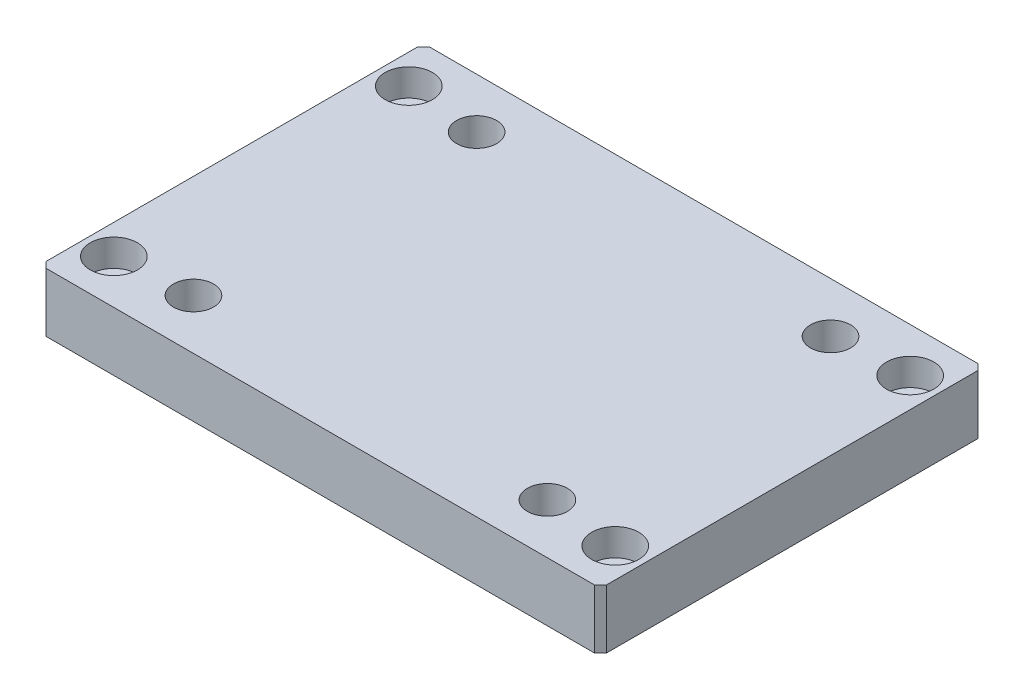
SolidWorks part; units mm, degrees
material "A6061"
ref_plane "前基準面" through (0, 0, 0) normal (0, 0, 1) x (1, 0, 0)
ref_plane "上基準面" through (0, 0, 0) normal (0, 1, 0) x (1, 0, 0)
ref_plane "右基準面" through (0, 0, 0) normal (1, 0, 0) x (0, 0, -1)
sketch "草图1" plane through (0, 0, 0) normal (0, 1, 0) x (1, 0, 0)
  line L1 (-47.5, -32.5) -> (47.5, -32.5)
  line L2 (-47.5, -32.5) -> (-47.5, 32.5)
  line L3 (-47.5, 32.5) -> (47.5, 32.5)
  line L4 (47.5, -32.5) -> (47.5, 32.5)
  line L5 (-47.5, -32.5) -> (47.5, 32.5) construction
  line L6 (-47.5, 32.5) -> (47.5, -32.5) construction
  point P0 (0, 0)
  dimension "D1" = 95
  dimension "D2" = 65
extrude "凸台-拉伸1" add sketch "草图1" along normal mid plane 10
chamfer "倒角1" distance 1 angle 45 4 edges at (47.5, 0, -32.5) (47.5, 0, 32.5) (-47.5, 0, 32.5) (-47.5, 0, -32.5)
sketch "草图2" plane through (0, 5, 0) normal (0, 1, 0) x (1, 0, 0)
  line L0 (0, 50.3233) -> (0, 0) construction
  line L1 (0, 0) -> (-46.7501, 0) construction
  point P0 (-42.5, 25)
  point P9 (-42.5, -25)
  point P10 (42.5, -25)
  point P11 (42.5, 25)
  dimension "D1" = 85
  dimension "D2" = 50
hole_wizard "M4 六角圆柱头螺钉的柱形沉头孔1" positions "草图2" profile "草图3" counterbore size "M4" standard "GB" end condition through all
sketch "草图3" plane through (-42.5, 5, -25) normal (1, 0, 0) x (0, 0, 1)
  line L0 (0, 0) -> (0, 10)
  line L1 (0, 10) -> (2.25, 10)
  line L3 (2.25, 10) -> (2.25, 4.6)
  line L4 (2.25, 4.6) -> (4, 4.6)
  line L5 (4, 4.6) -> (4, 0)
  line L7 (4, 0) -> (0, 0)
  line L11 (0, -6.35) -> (0, 107.95) construction
  dimension "通孔孔直径" = 4.5
  dimension "通孔孔深度" = 10
  dimension "柱形沉头孔直径" = 8
  dimension "柱形沉头孔深度" = 4.6
sketch "草图4" plane through (0, 5, 0) normal (0, 1, 0) x (1, 0, 0)
  line L0 (0, 51.5415) -> (0, 0) construction
  line L1 (0, 0) -> (61.7365, 0) construction
  point P0 (30, 24)
  point P11 (30, -24)
  point P12 (-30, -24)
  point P13 (-30, 24)
  dimension "D1" = 60
  dimension "D2" = 48
hole_wizard "M8 螺纹孔1" positions "草图4" profile "草图5" tap size "M8" standard "GB" end condition through all
sketch "草图5" plane through (30, 5, -24) normal (1, 0, 0) x (0, 0, 1)
  line L0 (0, 0) -> (0, 10)
  line L1 (0, 10) -> (3.4, 10)
  line L2 (3.4, 10) -> (3.4, 0)
  line L5 (3.4, 0) -> (0, 0)
  line L11 (0, -6.35) -> (0, 107.95) construction
  dimension "通孔螺纹孔钻头直径" = 6.8
  dimension "通孔螺纹孔钻头深度" = 10
cosmetic thread "孔螺纹线1" parameters "D2"=8
cosmetic thread "孔螺纹线2" parameters "D2"=8
cosmetic thread "孔螺纹线3" parameters "D2"=8
cosmetic thread "孔螺纹线4" parameters "D2"=8
